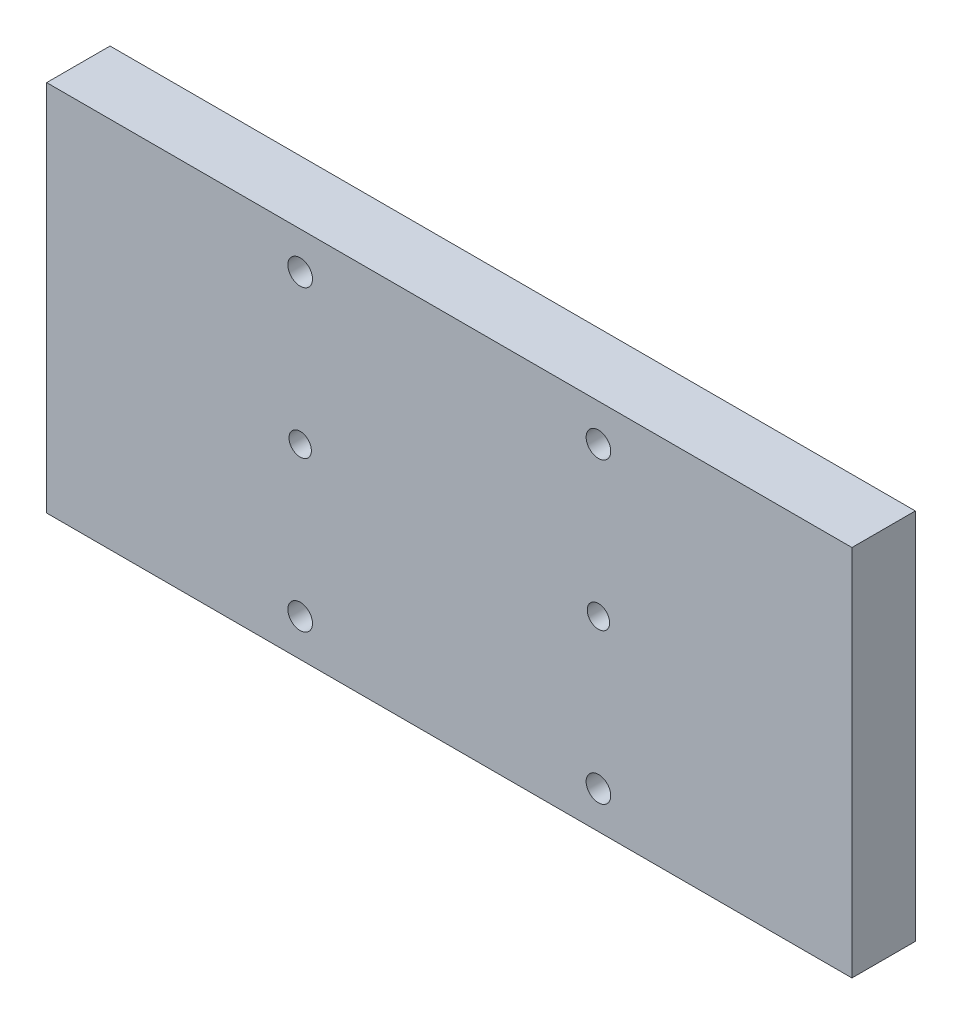
from build123d import *

# Parameters (mm, degrees)
SKETCH1_W                               = 216
SKETCH1_H                               = 100
BOSS_EXTRUDE1_DEPTH                     = 17
F_6_0_6_DIAMETER_HOLE1_D                = 6
CBORE_FOR_M6_HEX_HEAD_BOLT1_D           = 6.6
CBORE_FOR_M6_HEX_HEAD_BOLT1_CBORE_D     = 11
CBORE_FOR_M6_HEX_HEAD_BOLT1_CBORE_DEPTH = 6.8


with BuildPart() as part:
    # Sketch1 → Boss-Extrude1 (new body)
    with BuildSketch(Plane(origin=(0, 0, 0), x_dir=(-1, 0, 0), z_dir=(0, 0, -1))):
        Rectangle(SKETCH1_W, SKETCH1_H)
    extrude(amount=-BOSS_EXTRUDE1_DEPTH)

    # Ø6.0 (6) Diameter Hole1 (through all)
    with Locations(Plane(origin=(0, 0, 0), x_dir=(-1, 0, 0), z_dir=(0, 0, -1))):
        with Locations((-40, 0), (40, 0)):
            Hole(F_6_0_6_DIAMETER_HOLE1_D / 2)

    # CBORE for M6 Hex Head Bolt1 (through all)
    with Locations(Plane(origin=(0, 0, 0), x_dir=(-1, 0, 0), z_dir=(0, 0, -1))):
        with Locations((40, 40), (40, -40), (-40, -40), (-40, 40)):
            CounterBoreHole(CBORE_FOR_M6_HEX_HEAD_BOLT1_D / 2, CBORE_FOR_M6_HEX_HEAD_BOLT1_CBORE_D / 2, CBORE_FOR_M6_HEX_HEAD_BOLT1_CBORE_DEPTH)


solid = part.part
